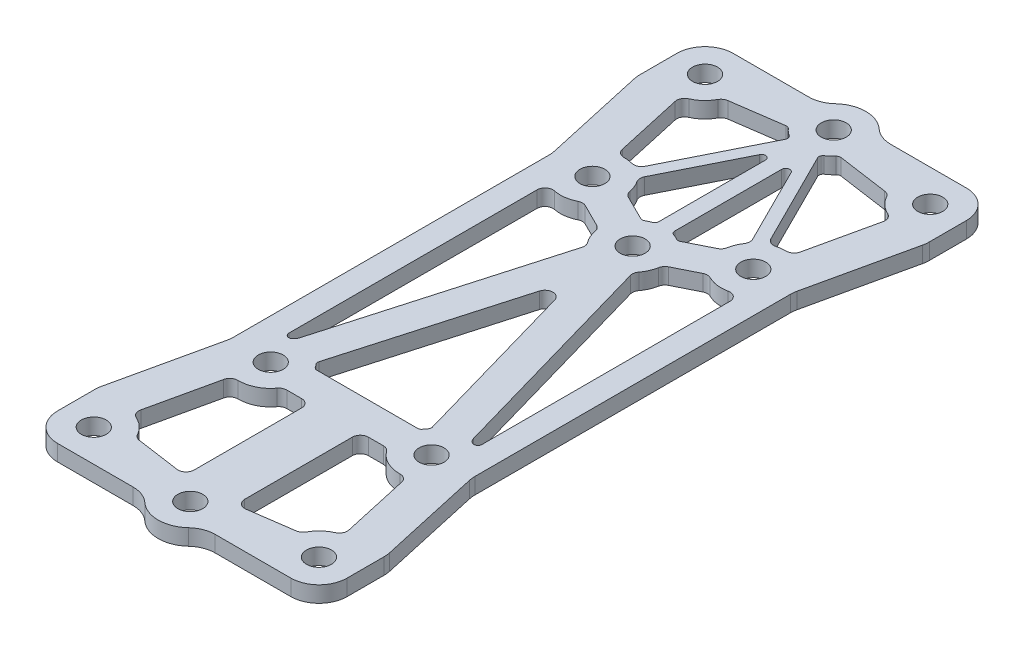
from build123d import *

# Parameters (mm, degrees)
SKETCH_3_R               = 1.55
EXTRUDE_1_DEPTH          = 2
CUT_EXTRUDE_1_DEPTH      = 48.581509013
CUT_EXTRUDE_1_DEPTH_BACK = 48.581509013
FILLET_1_R               = 3.5
FILLET_4_R               = 1
FILLET_5_R               = 0.5


with BuildPart() as part:
    # 草图3 → 凸台-拉伸1 (new body)
    # profile 1 of 7: a face of its own
    with BuildSketch(Plane(origin=(0, 0, 0), x_dir=(1, 0, 0), z_dir=(0, 1, 0))):
        with BuildLine():
            Line((-18, 42), (-18, -42))
            Line((-18, -42), (-3.464101615, -42))
            ThreePointArc((-3.464101615, -42), (-1.03527618, -36.136296695), (4, -40))
            ThreePointArc((4, -40), (3.863703305, -41.03527618), (3.464101615, -42))
            Line((3.464101615, -42), (18, -42))
            Line((18, -42), (18, 42))
            Line((18, 42), (3.464101615, 42))
            ThreePointArc((3.464101615, 42), (3.863703305, 41.03527618), (4, 40))
            ThreePointArc((4, 40), (-1.03527618, 36.136296695), (-3.464101615, 42))
            Line((-3.464101615, 42), (-18, 42))
        make_face()
        with Locations(Location((-14, -38, 0), (0, 0, 270))):
            Circle(SKETCH_3_R, mode=Mode.SUBTRACT)
        with Locations(Location((-10, -20, 0), (0, 0, 270))):
            Circle(SKETCH_3_R, mode=Mode.SUBTRACT)
        with Locations(Location((14, -38, 0), (0, 0, 270))):
            Circle(SKETCH_3_R, mode=Mode.SUBTRACT)
        with Locations(Location((10, -20, 0), (0, 0, 270))):
            Circle(SKETCH_3_R, mode=Mode.SUBTRACT)
        with Locations(Location((-10, 20, 0), (0, 0, 270))):
            Circle(SKETCH_3_R, mode=Mode.SUBTRACT)
        with Locations(Location((-14, 38, 0), (0, 0, 270))):
            Circle(SKETCH_3_R, mode=Mode.SUBTRACT)
        with Locations(Location((0, 15, 0), (0, 0, 270))):
            Circle(SKETCH_3_R, mode=Mode.SUBTRACT)
        with Locations(Location((10, 20, 0), (0, 0, 270))):
            Circle(SKETCH_3_R, mode=Mode.SUBTRACT)
        with Locations(Location((14, 38, 0), (0, 0, 270))):
            Circle(SKETCH_3_R, mode=Mode.SUBTRACT)
    # profile 2 of 7: a face of its own
    with BuildSketch(Plane(origin=(0, 0, 0), x_dir=(1, 0, 0), z_dir=(0, 1, 0))):
        with BuildLine():
            Line((-18, 42), (-18, -42))
            Line((-18, -42), (-3.464101615, -42))
            ThreePointArc((-3.464101615, -42), (-1.03527618, -36.136296695), (4, -40))
            ThreePointArc((4, -40), (3.863703305, -41.03527618), (3.464101615, -42))
            Line((3.464101615, -42), (18, -42))
            Line((18, -42), (18, 42))
            Line((18, 42), (3.464101615, 42))
            ThreePointArc((3.464101615, 42), (3.863703305, 41.03527618), (4, 40))
            ThreePointArc((4, 40), (-1.03527618, 36.136296695), (-3.464101615, 42))
            Line((-3.464101615, 42), (-18, 42))
        make_face()
        with Locations(Location((-14, -38, 0), (0, 0, 270))):
            Circle(SKETCH_3_R, mode=Mode.SUBTRACT)
        with Locations(Location((-10, -20, 0), (0, 0, 270))):
            Circle(SKETCH_3_R, mode=Mode.SUBTRACT)
        with Locations(Location((14, -38, 0), (0, 0, 270))):
            Circle(SKETCH_3_R, mode=Mode.SUBTRACT)
        with Locations(Location((10, -20, 0), (0, 0, 270))):
            Circle(SKETCH_3_R, mode=Mode.SUBTRACT)
        with Locations(Location((-10, 20, 0), (0, 0, 270))):
            Circle(SKETCH_3_R, mode=Mode.SUBTRACT)
        with Locations(Location((-14, 38, 0), (0, 0, 270))):
            Circle(SKETCH_3_R, mode=Mode.SUBTRACT)
        with Locations(Location((0, 15, 0), (0, 0, 270))):
            Circle(SKETCH_3_R, mode=Mode.SUBTRACT)
        with Locations(Location((10, 20, 0), (0, 0, 270))):
            Circle(SKETCH_3_R, mode=Mode.SUBTRACT)
        with Locations(Location((14, 38, 0), (0, 0, 270))):
            Circle(SKETCH_3_R, mode=Mode.SUBTRACT)
    # profile 3 of 7: a face of its own
    with BuildSketch(Plane(origin=(0, 0, 0), x_dir=(1, 0, 0), z_dir=(0, 1, 0))):
        with BuildLine():
            Line((-18, 42), (-18, -42))
            Line((-18, -42), (-3.464101615, -42))
            ThreePointArc((-3.464101615, -42), (-1.03527618, -36.136296695), (4, -40))
            ThreePointArc((4, -40), (3.863703305, -41.03527618), (3.464101615, -42))
            Line((3.464101615, -42), (18, -42))
            Line((18, -42), (18, 42))
            Line((18, 42), (3.464101615, 42))
            ThreePointArc((3.464101615, 42), (3.863703305, 41.03527618), (4, 40))
            ThreePointArc((4, 40), (-1.03527618, 36.136296695), (-3.464101615, 42))
            Line((-3.464101615, 42), (-18, 42))
        make_face()
        with Locations(Location((-14, -38, 0), (0, 0, 270))):
            Circle(SKETCH_3_R, mode=Mode.SUBTRACT)
        with Locations(Location((-10, -20, 0), (0, 0, 270))):
            Circle(SKETCH_3_R, mode=Mode.SUBTRACT)
        with Locations(Location((14, -38, 0), (0, 0, 270))):
            Circle(SKETCH_3_R, mode=Mode.SUBTRACT)
        with Locations(Location((10, -20, 0), (0, 0, 270))):
            Circle(SKETCH_3_R, mode=Mode.SUBTRACT)
        with Locations(Location((-10, 20, 0), (0, 0, 270))):
            Circle(SKETCH_3_R, mode=Mode.SUBTRACT)
        with Locations(Location((-14, 38, 0), (0, 0, 270))):
            Circle(SKETCH_3_R, mode=Mode.SUBTRACT)
        with Locations(Location((0, 15, 0), (0, 0, 270))):
            Circle(SKETCH_3_R, mode=Mode.SUBTRACT)
        with Locations(Location((10, 20, 0), (0, 0, 270))):
            Circle(SKETCH_3_R, mode=Mode.SUBTRACT)
        with Locations(Location((14, 38, 0), (0, 0, 270))):
            Circle(SKETCH_3_R, mode=Mode.SUBTRACT)
    # profile 4 of 7: a face of its own
    with BuildSketch(Plane(origin=(0, 0, 0), x_dir=(1, 0, 0), z_dir=(0, 1, 0))):
        with BuildLine():
            Line((3.464101615, 42), (-3.464101615, 42))
            ThreePointArc((-3.464101615, 42), (-1.03527618, 36.136296695), (4, 40))
            ThreePointArc((4, 40), (3.863703305, 41.03527618), (3.464101615, 42))
        make_face()
        with Locations(Location((0, 40, 0), (0, 0, 270))):
            Circle(SKETCH_3_R, mode=Mode.SUBTRACT)
    # profile 5 of 7: a face of its own
    with BuildSketch(Plane(origin=(0, 0, 0), x_dir=(1, 0, 0), z_dir=(0, 1, 0))):
        with BuildLine():
            ThreePointArc((3.464101615, 42), (0, 44), (-3.464101615, 42))
            Line((-3.464101615, 42), (3.464101615, 42))
        make_face()
    # profile 6 of 7: a face of its own
    with BuildSketch(Plane(origin=(0, 0, 0), x_dir=(1, 0, 0), z_dir=(0, 1, 0))):
        with BuildLine():
            Line((3.464101615, -42), (-3.464101615, -42))
            ThreePointArc((-3.464101615, -42), (0, -44), (3.464101615, -42))
        make_face()
    # profile 7 of 7: a face of its own
    with BuildSketch(Plane(origin=(0, 0, 0), x_dir=(1, 0, 0), z_dir=(0, 1, 0))):
        with BuildLine():
            ThreePointArc((4, -40), (-1.03527618, -36.136296695), (-3.464101615, -42))
            Line((-3.464101615, -42), (3.464101615, -42))
            ThreePointArc((3.464101615, -42), (3.863703305, -41.03527618), (4, -40))
        make_face()
        with Locations(Location((0, -40, 0), (0, 0, 270))):
            Circle(SKETCH_3_R, mode=Mode.SUBTRACT)
    extrude(amount=EXTRUDE_1_DEPTH)

    # 草图4 → 切除-拉伸1 (cut, two sides: drawn at the far end of the back side and taken through both)
    with BuildSketch(Plane(origin=(0, 2, 0), x_dir=(1, 0, 0), z_dir=(0, 1, 0)).offset(-CUT_EXTRUDE_1_DEPTH_BACK)):
        with BuildLine():
            ThreePointArc((-10.287871648, 36.509998961), (-11.411272912, 34.95065711), (-13.132278169, 34.095251759))
            Line((-13.132278169, 34.095251759), (-10.867721831, 23.904748241))
            ThreePointArc((-10.867721831, 23.904748241), (-9.511266945, 23.970030227), (-8.211145618, 23.577708764))
            Line((-8.211145618, 23.577708764), (-1.788854382, 36.422291236))
            ThreePointArc((-1.788854382, 36.422291236), (-2.529062482, 36.90099323), (-3.146442927, 37.530203064))
            Line((-3.146442927, 37.530203064), (-10.287871648, 36.509998961))
        make_face()
        Polygon((-15, 20), (-18, 33.5), (-18, -33.5), (-15, -20), align=None)
        with BuildLine():
            Line((-1, 34.645898034), (-7.000046818, 22.645804397))
            ThreePointArc((-7.000046818, 22.645804397), (-6.302422521, 21.525752532), (-6.007186132, 20.239661044))
            Line((-6.007186132, 20.239661044), (-2.203959486, 18.33804772))
            ThreePointArc((-2.203959486, 18.33804772), (-1.624154589, 18.655423624), (-1, 18.872983346))
            Line((-1, 18.872983346), (-1, 34.645898034))
        make_face()
        with BuildLine():
            Line((-12, 16.535898385), (-12, -16.535898385))
            ThreePointArc((-12, -16.535898385), (-11.500193455, -16.291979019), (-10.971385992, -16.119741084))
            Line((-10.971385992, -16.119741084), (-2.874709798, 12.218625596))
            ThreePointArc((-2.874709798, 12.218625596), (-3.661392772, 13.389347036), (-3.992813868, 14.760338956))
            Line((-3.992813868, 14.760338956), (-7.796040514, 16.66195228))
            ThreePointArc((-7.796040514, 16.66195228), (-9.880115622, 16.001796937), (-12, 16.535898385))
        make_face()
        with BuildLine():
            ThreePointArc((3.146442927, 37.530203064), (2.529062482, 36.90099323), (1.788854382, 36.422291236))
            Line((1.788854382, 36.422291236), (8.211145618, 23.577708764))
            ThreePointArc((8.211145618, 23.577708764), (9.511266945, 23.970030227), (10.867721831, 23.904748241))
            Line((10.867721831, 23.904748241), (13.132278169, 34.095251759))
            ThreePointArc((13.132278169, 34.095251759), (11.411272912, 34.95065711), (10.287871648, 36.509998961))
            Line((10.287871648, 36.509998961), (3.146442927, 37.530203064))
        make_face()
        Polygon((18, -33.5), (18, 33.5), (15, 20), (15, -20), align=None)
        with BuildLine():
            ThreePointArc((-6.535898385, -22), (-8.389933709, -23.661650794), (-10.867721831, -23.904748241))
            Line((-10.867721831, -23.904748241), (-13.132278169, -34.095251759))
            ThreePointArc((-13.132278169, -34.095251759), (-11.411272912, -34.95065711), (-10.287871648, -36.509998961))
            Line((-10.287871648, -36.509998961), (-3.146442927, -37.530203064))
            Line((-3.146442927, -37.530203064), (-3.146442927, -22))
            Line((-3.146442927, -22), (-6.535898385, -22))
        make_face()
        with BuildLine():
            ThreePointArc((6.007186132, 20.239661044), (6.302422521, 21.525752532), (7.000046818, 22.645804397))
            Line((7.000046818, 22.645804397), (1, 34.645898034))
            Line((1, 34.645898034), (1, 18.872983346))
            ThreePointArc((1, 18.872983346), (1.624154589, 18.655423624), (2.203959486, 18.33804772))
            Line((2.203959486, 18.33804772), (6.007186132, 20.239661044))
        make_face()
        with BuildLine():
            Line((0, 7.719890111), (-7.125290202, -17.218625596))
            ThreePointArc((-7.125290202, -17.218625596), (-6.806605408, -17.591217947), (-6.535898385, -18))
            Line((-6.535898385, -18), (6.535898385, -18))
            ThreePointArc((6.535898385, -18), (6.806605408, -17.591217947), (7.125290202, -17.218625596))
            Line((7.125290202, -17.218625596), (0, 7.719890111))
        make_face()
        with BuildLine():
            Line((12, -16.535898385), (12, 16.535898385))
            ThreePointArc((12, 16.535898385), (9.880115622, 16.001796937), (7.796040514, 16.66195228))
            Line((7.796040514, 16.66195228), (3.992813868, 14.760338956))
            ThreePointArc((3.992813868, 14.760338956), (3.661392772, 13.389347036), (2.874709798, 12.218625596))
            Line((2.874709798, 12.218625596), (10.971385992, -16.119741084))
            ThreePointArc((10.971385992, -16.119741084), (11.500193455, -16.291979019), (12, -16.535898385))
        make_face()
        with BuildLine():
            ThreePointArc((10.287871648, -36.509998961), (11.411272912, -34.95065711), (13.132278169, -34.095251759))
            Line((13.132278169, -34.095251759), (10.867721831, -23.904748241))
            ThreePointArc((10.867721831, -23.904748241), (8.389933709, -23.661650794), (6.535898385, -22))
            Line((6.535898385, -22), (3.146442927, -22))
            Line((3.146442927, -22), (3.146442927, -37.530203064))
            Line((3.146442927, -37.530203064), (10.287871648, -36.509998961))
        make_face()
    extrude(amount=CUT_EXTRUDE_1_DEPTH + CUT_EXTRUDE_1_DEPTH_BACK, mode=Mode.SUBTRACT)

    # 圆角1
    fillet_1_edges = [part.edges().sort_by_distance(p)[0] for p in [
        (-18, 1, -33.5),
        (-15, 1, -20),
        (-15, 1, 20),
        (-18, 1, 33.5),
        (15, 1, 20),
        (15, 1, -20),
        (18, 1, -33.5),
        (18, 1, 33.5),
        (-18, 1, 42),
        (-18, 1, -42),
        (-3.464101615, 1, -42),
        (3.464101615, 1, -42),
        (18, 1, -42),
        (18, 1, 42),
        (3.464101615, 1, 42),
        (-3.464101615, 1, 42),
    ]]
    fillet(fillet_1_edges, radius=FILLET_1_R)

    # 圆角4
    fillet_4_edges = [part.edges().sort_by_distance(p)[0] for p in [
        (7.796040514, 1, -16.66195228),
        (12, 1, -16.535898385),
        (10.971385992, 1, 16.119741084),
        (2.874709798, 1, -12.218625596),
        (3.992813868, 1, -14.760338956),
        (-3.992813868, 1, -14.760338956),
        (-2.874709798, 1, -12.218625596),
        (-10.971385992, 1, 16.119741084),
        (-12, 1, -16.535898385),
        (-7.796040514, 1, -16.66195228),
        (13.132278169, 1, 34.095251759),
        (10.287871648, 1, 36.509998961),
        (3.146442927, 1, 37.530203064),
        (3.146442927, 1, 22),
        (6.535898385, 1, 22),
        (10.867721831, 1, 23.904748241),
        (-10.287871648, 1, 36.509998961),
        (-13.132278169, 1, 34.095251759),
        (-10.867721831, 1, 23.904748241),
        (-6.535898385, 1, 22),
        (-3.146442927, 1, 22),
        (-3.146442927, 1, 37.530203064),
        (-6.007186132, 1, -20.239661044),
        (-7.000046818, 1, -22.645804397),
        (10.867721831, 1, -23.904748241),
        (8.211145618, 1, -23.577708764),
        (10.287871648, 1, -36.509998961),
        (13.132278169, 1, -34.095251759),
        (7.000046818, 1, -22.645804397),
        (6.007186132, 1, -20.239661044),
        (0, 1, -7.719890111),
        (-8.211145618, 1, -23.577708764),
        (-10.867721831, 1, -23.904748241),
        (-13.132278169, 1, -34.095251759),
        (-10.287871648, 1, -36.509998961),
    ]]
    fillet(fillet_4_edges, radius=FILLET_4_R)

    # 圆角5
    fillet_5_edges = [part.edges().sort_by_distance(p)[0] for p in [
        (-7.125290202, 1, 17.218625596),
        (-6.535898385, 1, 18),
        (6.535898385, 1, 18),
        (7.125290202, 1, 17.218625596),
        (12, 1, 16.535898385),
        (-12, 1, 16.535898385),
        (2.203959486, 1, -18.33804772),
        (1, 1, -18.872983346),
        (-1, 1, -18.872983346),
        (-2.203959486, 1, -18.33804772),
        (1, 1, -34.645898034),
        (-1, 1, -34.645898034),
        (3.146442927, 1, -37.530203064),
        (1.788854382, 1, -36.422291236),
        (-1.788854382, 1, -36.422291236),
        (-3.146442927, 1, -37.530203064),
    ]]
    fillet(fillet_5_edges, radius=FILLET_5_R)


solid = part.part
